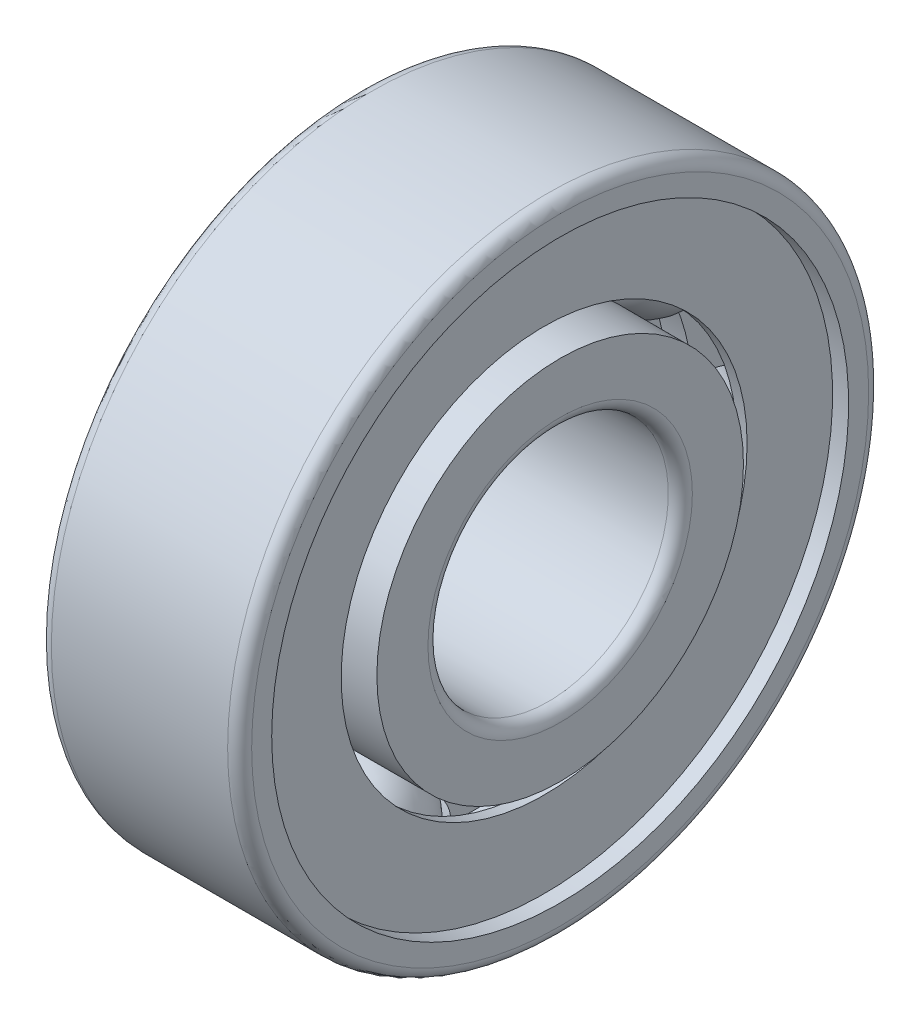
SolidWorks part; units mm, degrees
revolve "Boss-Revolve2" add sketch "Sketch6" angle 360 about L4
sketch "Sketch6" plane through (0, 0, 0) normal (0, 0, 1) x (1, 0, 0)
  line L0 (0, 0) -> (5.5439, 0) construction
  line L1 (-12.4206, 0) -> (9.8128, 0) construction
  line L2 (0, 0) -> (0, 11.4011) construction
  line L3 (-5.5681, 11.775) -> (6.1049, 11.775) construction
  line L4 (-5.5681, 11.775) -> (6.1049, 11.775) construction
  line L5 (-2.9765, 11.775) -> (2.9765, 11.775)
  arc A0 (-2.9765, 11.775) -> (2.9765, 11.775) centre (0, 11.775) ccw
  dimension "Dw" = 5.953
revolve "Base-Revolve" add sketch "Sketch2" angle 360 about L0
sketch "Sketch2" plane through (0, 0, 0) normal (0, 0, 1) x (1, 0, 0)
  line L0 (-12.4206, 0) -> (9.8128, 0) construction
  line L1 (0, 0) -> (0, 37.3563) construction
  line L2 (-5.5681, 11.775) -> (6.1049, 11.775) construction
  line L3 (-0.6548, 12.5935) -> (0.6548, 12.5935)
  line L4 (-0.6548, 12.5935) -> (-0.6548, 10.9565)
  line L5 (-0.6548, 10.9565) -> (0.6548, 10.9565)
  line L6 (0.6548, 12.5935) -> (0.6548, 10.9565)
  dimension "D1" = 1.3097
  dimension "D2" = 0.6548
  dimension "D3" = 1.6371
  dimension "D4" = 0.8185
  dimension "D5" = 11.775
revolve "Boss-Revolve1" add sketch "Sketch3" angle 360 about L1
sketch "Sketch3" plane through (0, 0, 0) normal (0, 0, 1) x (1, 0, 0)
  line L0 (-5.5681, 11.775) -> (6.1049, 11.775) construction
  line L1 (-5.5681, 11.775) -> (6.1049, 11.775) construction
  line L2 (-12.4206, 0) -> (9.8128, 0) construction
  line L3 (-12.4206, 0) -> (9.8128, 0) construction
  line L4 (0, 0) -> (0, 37.3563) construction
  line L5 (0, 0) -> (0, 37.3563) construction
  line L6 (-3.2741, 11.775) -> (3.2741, 11.775)
  arc A0 (-3.2741, 11.775) -> (3.2741, 11.775) centre (0, 11.775) ccw
  dimension "Dwww" = 6.5483
  dimension "D2" = 3.2741
pattern_circular "CirPattern1" count 7 over 360 about axis through (0, 0, 0) along (1, 0, 0) of "Boss-Revolve1"
revolve "Boss-Revolve3" add sketch "Sketch7" angle 360 about L0
sketch "Sketch7" plane through (0, 0, 0) normal (0, 0, 1) x (1, 0, 0)
  line L0 (0, 0) -> (6.6488, 0) construction
  line L1 (0, 0) -> (0, 16.8954) construction
  line L2 (-4.4, 16) -> (4.4, 16)
  line L3 (-5, 15.4) -> (-5, 14.4)
  line L4 (-5, 14.4) -> (-1.3818, 14.4)
  line L5 (5, 15.4) -> (5, 14.4)
  line L6 (1.3818, 14.4) -> (3.6648, 14.4)
  line L7 (4.2, 14.4) -> (5, 14.4)
  line L8 (3.6648, 14) -> (4.2, 14)
  line L9 (3.6648, 14) -> (3.6648, 14.4)
  line L11 (4.2, 14) -> (4.2, 14.4)
  arc A0 (-4.4, 16) -> (-5, 15.4) centre (-4.4, 15.4) ccw
  arc A1 (4.4, 16) -> (5, 15.4) centre (4.4, 15.4) cw
  arc A2 (2.8617, 12.5935) -> (-2.8617, 12.5935) centre (0, 11.775) ccw construction
  arc A3 (1.4032, 14.4) -> (-0.0003, 8.7985) centre (0, 11.775) ccw construction
  arc A4 (1.3818, 14.4) -> (-1.3818, 14.4) centre (0, 11.775) ccw
  point P10 (-5, 16)
  point P13 (5, 16)
ref_plane "Plane1" through (0, 0, 0) normal (0, 0, 1) x (1, 0, 0)
ref_plane "Plane2" through (0, 0, 0) normal (0, 1, 0) x (1, 0, 0)
ref_plane "Plane3" through (0, 0, 0) normal (1, 0, 0) x (0, 0, -1)
sketch "Dimension sketch" plane through (0, 0, 0) normal (0, 0, 1) x (1, 0, 0)
  point P0 (0, -75.4307)
  point P1 (5.953, -75.4307)
  point P2 (0, 50.7088)
  point P3 (12, 50.7088)
  point P4 (32, 50.7088)
  point P5 (10, 50.7088)
  point P6 (0, -10.9899)
  point P7 (18.3, -10.9899)
  point P8 (28, -10.9899)
  point P9 (0.6, -10.9899)
  point P10 (7, -75.4307)
sketch "Sketch4" plane through (0, 0, 0) normal (0, 0, 1) x (1, 0, 0)
  line L0 (0, 0) -> (8.1272, 0) construction
  line L1 (-12.4206, 0) -> (9.8128, 0) construction
  line L3 (-0.6548, 12.5935) -> (0.6548, 12.5935) construction
  line L4 (-3.2742, 15.8677) -> (3.2741, 15.8677)
  line L5 (-3.2742, 15.8677) -> (-3.2742, 12.5935)
  line L6 (-3.2742, 12.5935) -> (3.2741, 12.5935)
  line L7 (3.2741, 15.8677) -> (3.2741, 12.5935)
revolve "Cut-Revolve1" cut sketch "Sketch4" angle 360 about L0
sketch "Sketch5" plane through (0, 0, 0) normal (0, 0, 1) x (1, 0, 0)
  line L0 (0, 0) -> (8.2665, 0) construction
  line L1 (-12.4206, 0) -> (9.8128, 0) construction
  line L2 (-0.6548, 10.9565) -> (0.6548, 10.9565) construction
  line L3 (-3.2742, 10.9565) -> (3.2741, 10.9565)
  line L4 (-3.2742, 10.9565) -> (-3.2742, 7.6823)
  line L5 (-3.2742, 7.6823) -> (3.2741, 7.6823)
  line L6 (3.2741, 10.9565) -> (3.2741, 7.6823)
revolve "Cut-Revolve2" cut sketch "Sketch5" angle 360 about L0
pattern_circular "CirPattern2" count 7 over 360 about axis through (0, 0, 0) along (1, 0, 0) of "Boss-Revolve2"
sketch "Sketch8" plane through (0, 0, 0) normal (0, 0, 1) x (1, 0, 0)
  line L0 (-12.4206, 0) -> (9.8128, 0) construction
  line L1 (-12.4206, 0) -> (9.8128, 0) construction
  line L2 (5, 15.4) -> (5, 14.4) construction
  line L3 (-5, 9.15) -> (-1.3818, 9.15)
  line L4 (-5, 9.15) -> (-5, 6.6)
  line L5 (-4.4, 6) -> (4.4, 6)
  line L6 (5, 9.15) -> (5, 6.6)
  line L7 (-5, 15.4) -> (-5, 14.4) construction
  line L8 (1.3818, 9.15) -> (5, 9.15)
  arc A0 (-5, 6.6) -> (-4.4, 6) centre (-4.4, 6.6) ccw
  arc A1 (4.4, 6) -> (5, 6.6) centre (4.4, 6.6) ccw
  arc A2 (-2.8617, 10.9565) -> (2.8617, 10.9565) centre (0, 11.775) ccw construction
  arc A3 (-2.8617, 10.9565) -> (2.8617, 10.9565) centre (0, 11.775) ccw construction
  arc A4 (-1.3818, 9.15) -> (1.3818, 9.15) centre (0, 11.775) ccw
revolve "Boss-Revolve4" add sketch "Sketch8" angle 360 about L1
sketch "Sketch10" plane through (0, 0, 0) normal (0, 0, 1) x (1, 0, 0)
  line L0 (3.6648, 14.4) -> (3.6648, -14.4) construction
  line L1 (4.2, 14) -> (3.6648, 14)
  line L2 (4.2, 14) -> (4.2, 10.1322)
  line L3 (4.2, 10.1322) -> (3.6648, 10.1322)
  line L4 (3.6648, 14) -> (3.6648, 10.1322)
  line L5 (1.3818, 9.15) -> (5, 9.15) construction
  line L6 (0, 0) -> (-5.3515, 0) construction
  line L7 (-12.4206, 0) -> (9.8128, 0) construction
revolve "Boss-Revolve5" add sketch "Sketch10" angle 360 about L6
sketch "Sketch11" plane through (0, 0, 0) normal (1, 0, 0) x (0, 0, -1)
  circle A0 centre (0, 0) radius 16
  circle A1 centre (0, 0) radius 16 construction
extrude "Cut-Extrude1" cut sketch "Sketch11" against normal blind 10
mirror "Mirror All1" about plane through (0, 0, 0) normal (1, 0, 0) of bodies 109
equation "\"D5@Sketch7\" = \"防尘圈径D3@Dimension sketch\""
equation "\"Z@CirPattern1\"=\"球数Z@Dimension sketch\" "
equation "\"Dw@Sketch6\"=\"球径DW@Dimension sketch\""
equation "\"DD@Sketch8\"=\"d@Dimension sketch\""
equation "\"D@Sketch7\"=\"DD@Dimension sketch\""
equation "\"B@Sketch7\"=\"B@Dimension sketch\" "
equation "\"DD2@Sketch8\"=\"内圈外径DD2@Dimension sketch\""
equation "\"R@Sketch7\"=\"r@Dimension sketch\""
equation "\"D3@Sketch2\" = 0.25*\"Dwww@Sketch3\""
equation "\"D4@Sketch2\" = \"D3@Sketch2\"/2"
equation "\"Dwww@Sketch3\" = 1.1*\"Dw@Sketch6\""
equation "\"D2@Sketch3\" = 0.5*\"Dwww@Sketch3\""
equation "\"D1@Sketch2\" = 0.2*\"Dwww@Sketch3\""
equation "\"D2@Sketch2\" = 0.5*\"D1@Sketch2\""
equation "\"切除位置@Sketch4\" = \"Dwww@Sketch3\"/2"
equation "\"D1@CirPattern2\" = \"Z@CirPattern1\""
equation "\"D3@Sketch7\" = \"B@Sketch7\" / 2"
equation "\"D1@Sketch8\" = \"R@Sketch7\""
equation "\"D2@Sketch7\" = 0.9*\"D@Sketch7\""
equation "\"D5@Sketch2\" = 0.25* ( \"D2@Sketch7\" + \"DD2@Sketch8\" )  "
equation "\"D6@Sketch7\" = 0.08 * \"B@Sketch7\""
equation "\"D1@Sketch10\" = 0.15*\"Dwww@Sketch3\""
